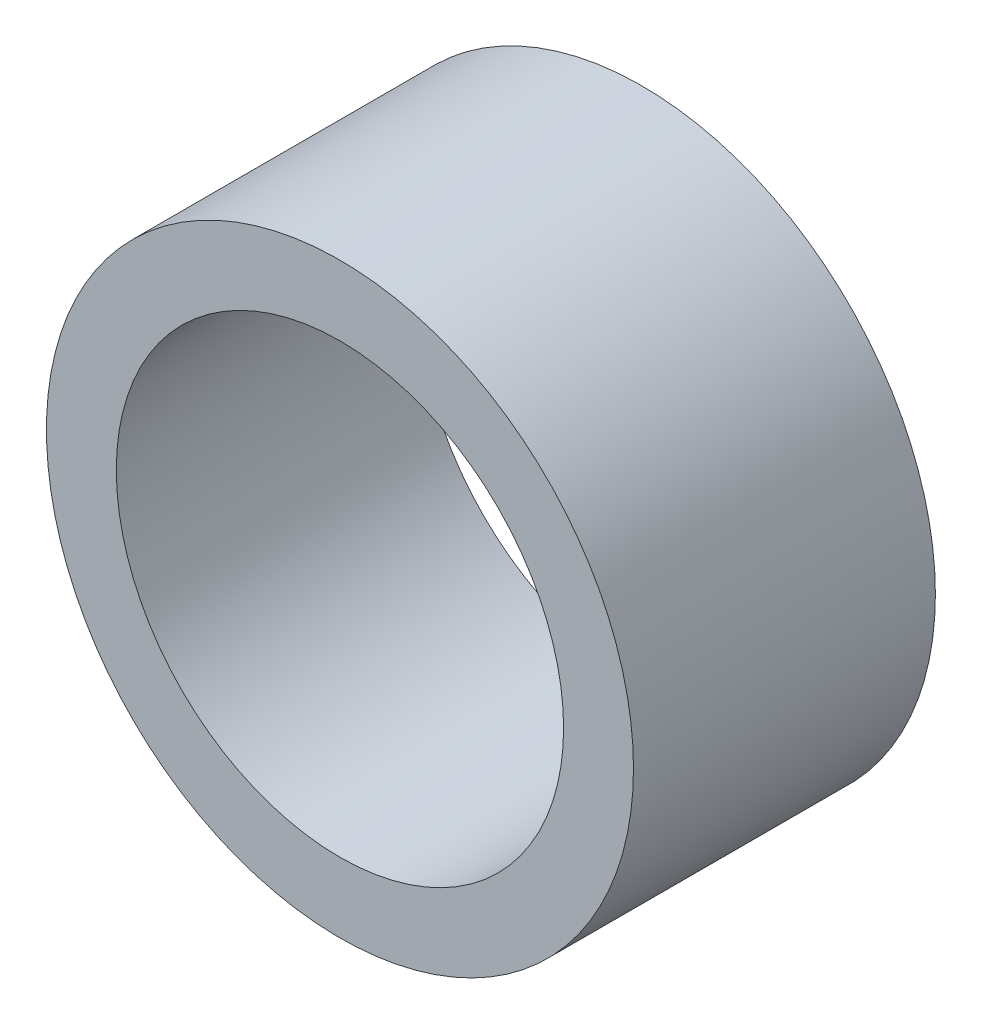
from build123d import *

# Parameters (mm, degrees)
SKETCH_1_R          = 210
EXTRUDE_1_DEPTH     = 216
SKETCH_2_R          = 160
CUT_EXTRUDE_1_DEPTH = 250


with BuildPart() as part:
    # 草图1 → 凸台-拉伸1 (new body)
    with BuildSketch(Plane.XY):
        Circle(SKETCH_1_R)
    extrude(amount=EXTRUDE_1_DEPTH)

    # 草图2 → 切除-拉伸1 (cut)
    with BuildSketch(Plane.XY):
        Circle(SKETCH_2_R)
    extrude(amount=CUT_EXTRUDE_1_DEPTH, mode=Mode.SUBTRACT)


solid = part.part
